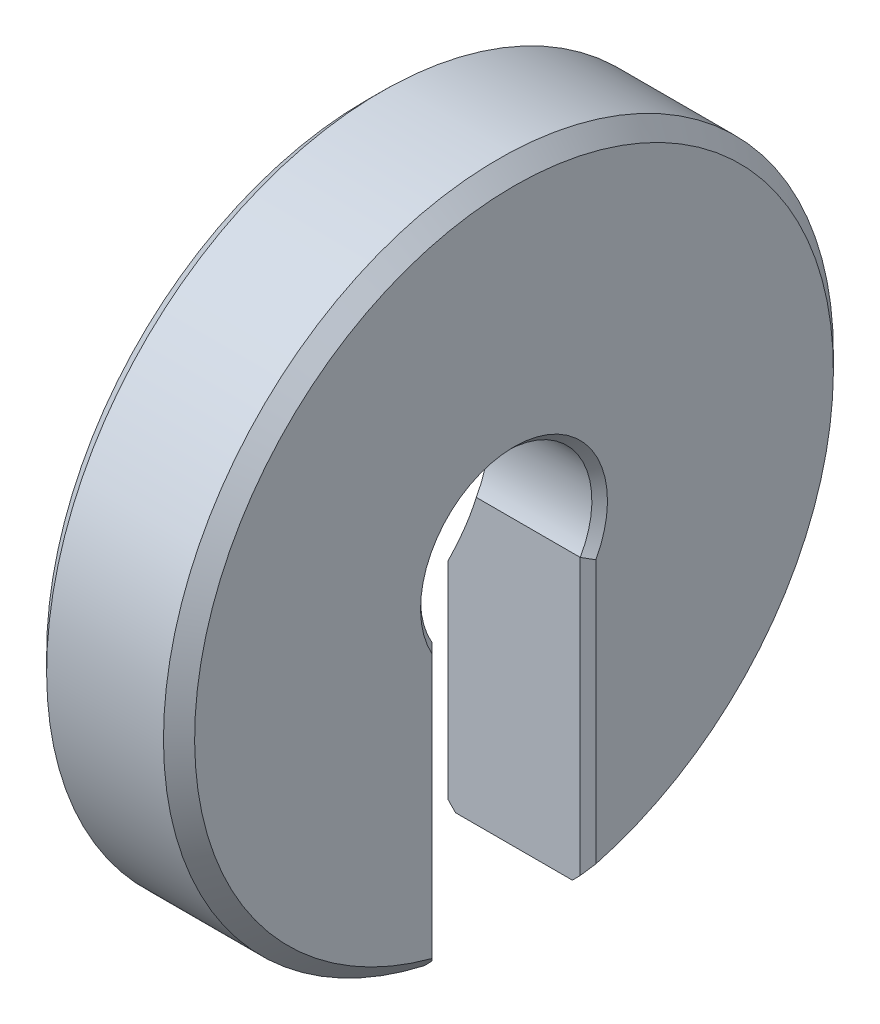
SolidWorks part; units mm, degrees
ref_plane "Front Plane" through (0, 0, 0) normal (0, 0, 1) x (1, 0, 0)
ref_plane "Top Plane" through (0, 0, 0) normal (0, 1, 0) x (1, 0, 0)
ref_plane "Right Plane" through (0, 0, 0) normal (1, 0, 0) x (0, 0, -1)
sketch "Sketch1" plane through (0, 0, 0) normal (0, 0, 1) x (1, 0, 0)
  line L0 (-44.9505, 0) -> (57.9006, 0) construction
  line L1 (-19, 19.05) -> (-19, 43)
  line L2 (-19, 43) -> (0, 43)
  line L3 (0, 43) -> (0, 11)
  line L4 (-14.35, 11) -> (0, 11)
  line L5 (-14.35, 11) -> (-19, 19.05)
  dimension "D1" = 19
  dimension "D2" = 43
  dimension "D3" = 11
  dimension "D4" = 19.05
  dimension "D5" = 4.65
revolve "Revolve1" add sketch "Sketch1" angle 360 about L0
chamfer "Chamfer1" distance 2 angle 45 2 edges at (0, 0, 43) (-19, 0, 43)
sketch "Sketch13" plane through (-19, 0, 0) normal (-1, 0, 0) x (0, 0, 1)
  line L1 (-9.5, 0) -> (-9.5, -65.514)
  line L2 (9.5, 0) -> (9.5, -73.6971)
  line L3 (-9.5, 0) -> (9.5, 0)
  line L4 (-9.5, -65.514) -> (9.5, -73.6971)
  dimension "D1" = 65.514
extrude "Cut-Extrude2" cut sketch "Sketch13" against normal blind 43
chamfer "Chamfer2" distance 1 angle 45 5 edges at (-19, -28.1982, -9.5) (-19, -28.1982, 9.5) (0, -22.7147, -9.5) (0, 11, 0) (0, -22.7147, 9.5)
